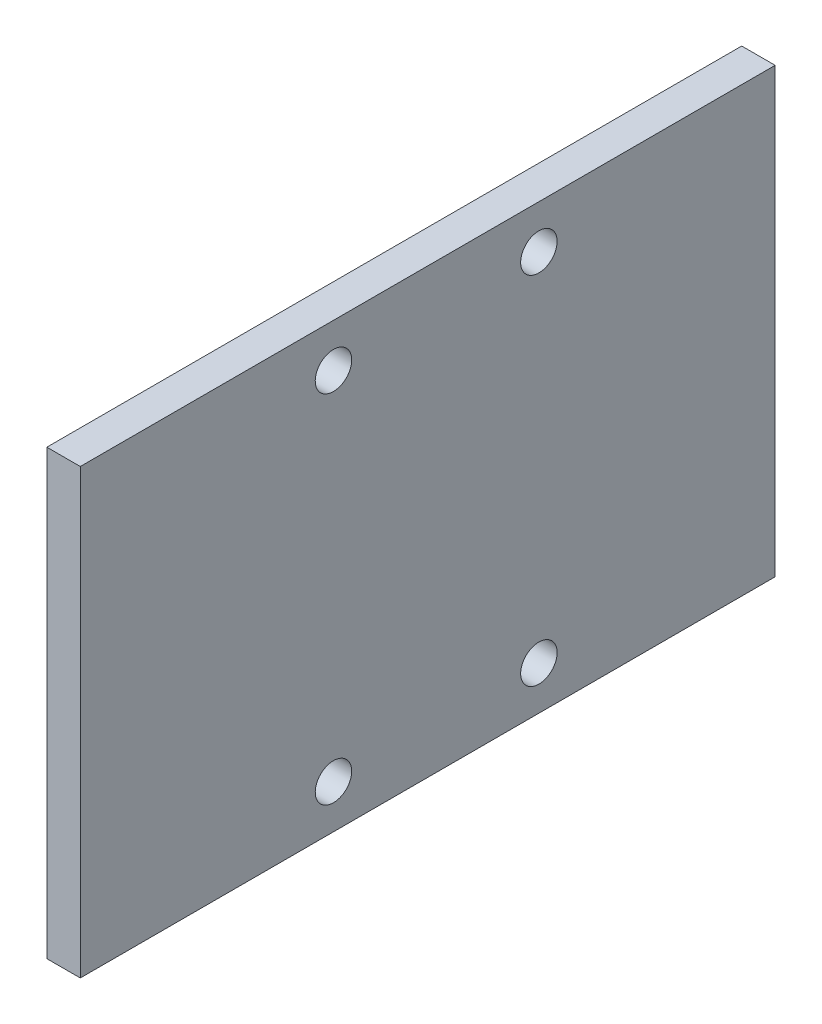
from build123d import *

# Parameters (mm, degrees)
SKETCH_1_W          = 3.85
SKETCH_1_H          = 51
EXTRUDE_1_DEPTH     = 80
CUT_EXTRUDE_1_REACH = 1465.749
SKETCH_2_R          = 2.1


with BuildPart() as part:
    # 草图1 → 凸台-拉伸1 (new body)
    with BuildSketch(Plane.XY):
        with Locations((-0.405329913, -17.044468303)):
            Rectangle(SKETCH_1_W, SKETCH_1_H)
    extrude(amount=EXTRUDE_1_DEPTH)

    # 草图2 → 切除-拉伸1 (cut, up to next)
    with BuildSketch(Plane(origin=(5.369670087, -1051.794731348, 1009.143932915), x_dir=(0, -1, 0), z_dir=(1, 0, 0)), mode=Mode.PRIVATE) as cut_extrude_1_sk1:
        with Locations((-1055.250263055, 981.942263912)):
            Circle(SKETCH_2_R)
    cut_extrude_1_tool1 = extrude(cut_extrude_1_sk1.sketch, amount=-CUT_EXTRUDE_1_REACH, mode=Mode.PRIVATE) & part.part
    # 草图2 → 切除-拉伸1 (cut, up to next)
    with BuildSketch(Plane(origin=(5.369670087, -1051.794731348, 1009.143932915), x_dir=(0, -1, 0), z_dir=(1, 0, 0)), mode=Mode.PRIVATE) as cut_extrude_1_sk2:
        with Locations((-1055.250263055, 958.292263912)):
            Circle(SKETCH_2_R)
    cut_extrude_1_tool2 = extrude(cut_extrude_1_sk2.sketch, amount=-CUT_EXTRUDE_1_REACH, mode=Mode.PRIVATE) & part.part
    # 草图2 → 切除-拉伸1 (cut, up to next)
    with BuildSketch(Plane(origin=(5.369670087, -1051.794731348, 1009.143932915), x_dir=(0, -1, 0), z_dir=(1, 0, 0)), mode=Mode.PRIVATE) as cut_extrude_1_sk3:
        with Locations((-1014.250263055, 958.292263912)):
            Circle(SKETCH_2_R)
    cut_extrude_1_tool3 = extrude(cut_extrude_1_sk3.sketch, amount=-CUT_EXTRUDE_1_REACH, mode=Mode.PRIVATE) & part.part
    # 草图2 → 切除-拉伸1 (cut, up to next)
    with BuildSketch(Plane(origin=(5.369670087, -1051.794731348, 1009.143932915), x_dir=(0, -1, 0), z_dir=(1, 0, 0)), mode=Mode.PRIVATE) as cut_extrude_1_sk4:
        with Locations((-1014.250263055, 981.942263912)):
            Circle(SKETCH_2_R)
    cut_extrude_1_tool4 = extrude(cut_extrude_1_sk4.sketch, amount=-CUT_EXTRUDE_1_REACH, mode=Mode.PRIVATE) & part.part
    add(cut_extrude_1_tool1.solids().sort_by_distance((5.36967, 3.455532, 27.201669))[0], mode=Mode.SUBTRACT)
    add(cut_extrude_1_tool2.solids().sort_by_distance((5.36967, 3.455532, 50.851669))[0], mode=Mode.SUBTRACT)
    add(cut_extrude_1_tool3.solids().sort_by_distance((5.36967, -37.544468, 50.851669))[0], mode=Mode.SUBTRACT)
    add(cut_extrude_1_tool4.solids().sort_by_distance((5.36967, -37.544468, 27.201669))[0], mode=Mode.SUBTRACT)


solid = part.part
